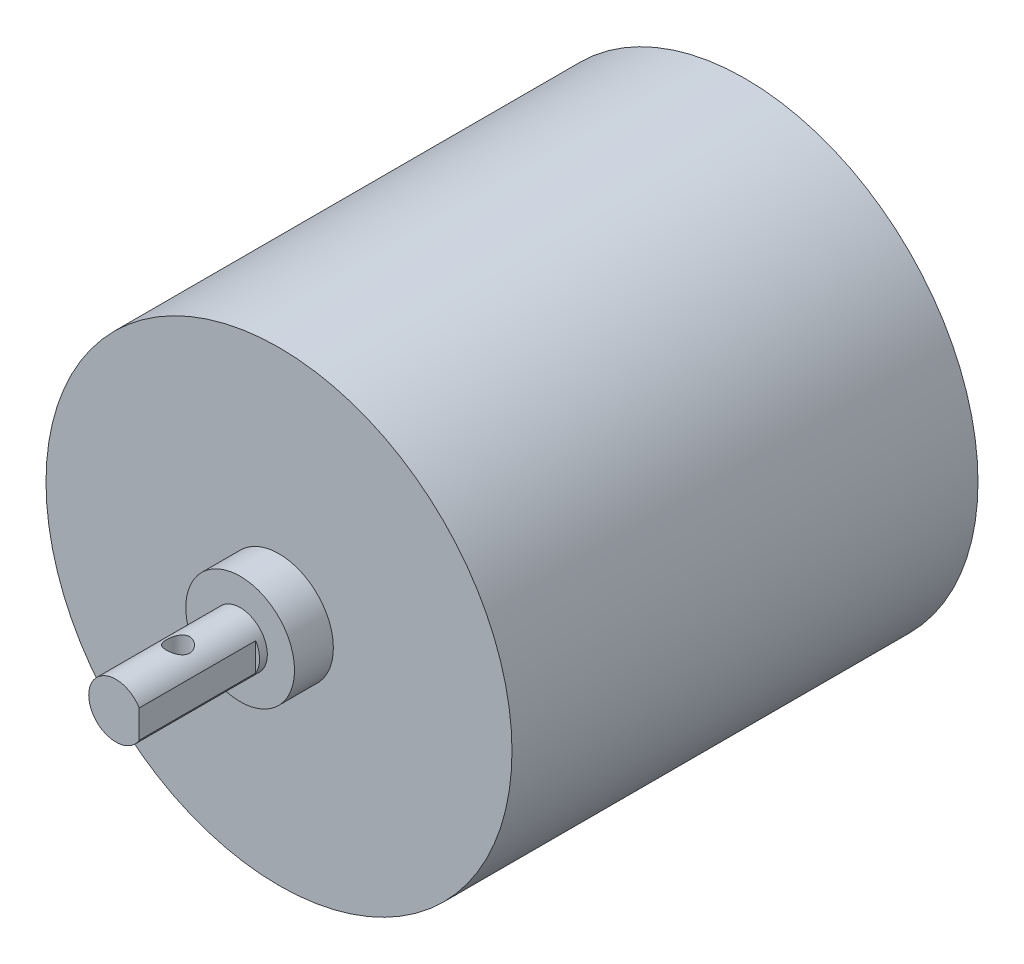
SolidWorks part; units mm, degrees
ref_plane "前视基准面" through (0, 0, 0) normal (0, 0, 1) x (1, 0, 0)
ref_plane "上视基准面" through (0, 0, 0) normal (0, 1, 0) x (1, 0, 0)
ref_plane "右视基准面" through (0, 0, 0) normal (1, 0, 0) x (0, 0, -1)
sketch "草图1" plane through (0, 0, 0) normal (0, 0, 1) x (1, 0, 0)
  circle A0 centre (0, 0) radius 30
  dimension "D1" = 60
extrude "凸台-拉伸1" add sketch "草图1" along normal blind 60
sketch "草图2" plane through (0, 0, 60) normal (0, 0, 1) x (1, 0, 0)
  circle A0 centre (0, 0) radius 7
  dimension "D1" = 14
extrude "凸台-拉伸2" add sketch "草图2" along normal blind 5
sketch "草图3" plane through (0, 0, 65) normal (0, 0, 1) x (1, 0, 0)
  circle A0 centre (0, 0) radius 3.5
  dimension "D1" = 7
extrude "凸台-拉伸3" add sketch "草图3" along normal blind 16
sketch "草图4" plane through (0, 0, 81) normal (0, 0, 1) x (1, 0, 0)
  line L0 (3, 1.8028) -> (3, -1.8028)
  line L1 (3, 0) -> (3.5, 0) construction
  circle A0 centre (0, 0) radius 3.5 construction
  circle A1 centre (0, 0) radius 3.5 construction
  circle A3 centre (0, 0) radius 3.5
  circle A4 centre (0, 0) radius 3.5
  circle M3 centre (0, 0) radius 3.5
  dimension "D1" = 0
  dimension "D2" = 0.5
extrude "切除-拉伸1" cut sketch "草图4" against normal blind 15 contours L0 L1 A4 | L1 L0 M3
sketch "草图5" plane through (3, 0, 0) normal (0, -1, 0) x (0, 0, -1)
  line L0 (-81, -3) -> (-73, -3) construction
  line L2 (-81, 0) -> (-81, -6.5) construction
  circle A0 centre (-73, -3) radius 1.5
  dimension "D1" = 3
  dimension "D2" = 8
  dimension "D3" = 3.5
extrude "切除-拉伸2" cut sketch "草图5" against normal mid plane 15
